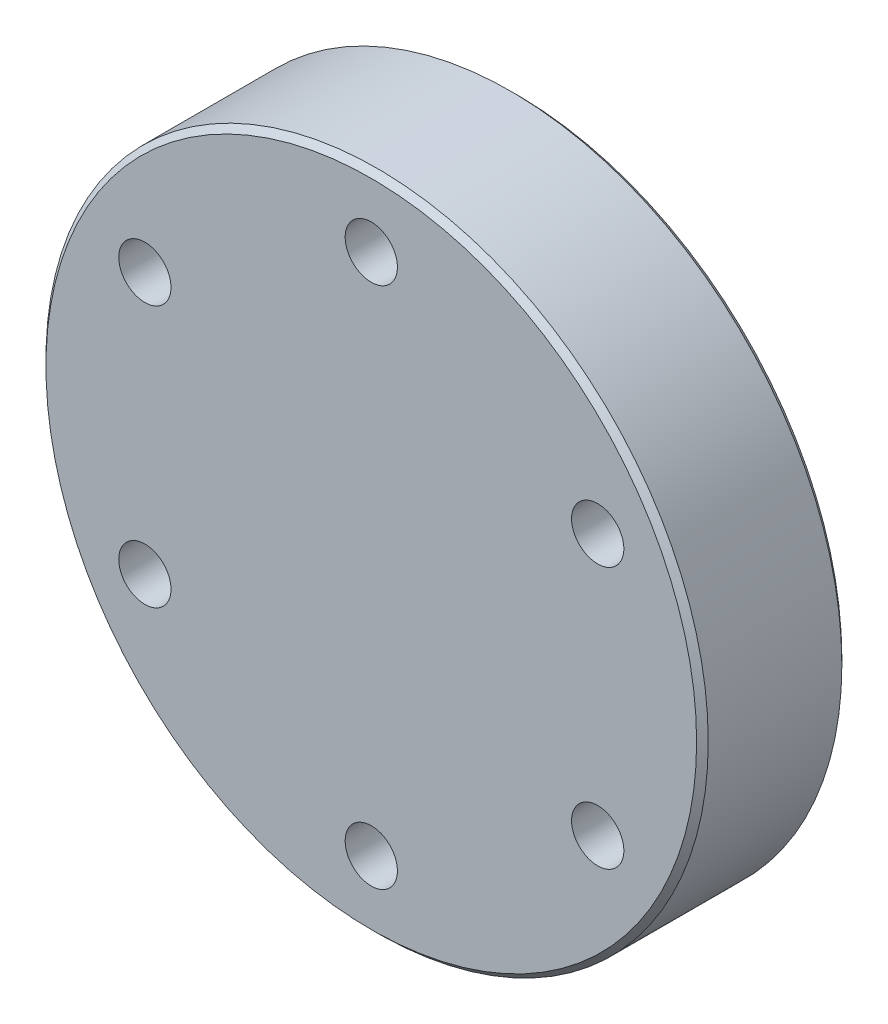
from build123d import *

# Parameters (mm, degrees)
SKETCH1_R                                           = 57
BOSS_EXTRUDE1_DEPTH                                 = 25
CHAMFER3_SIZE                                       = 1
HOLE_SIZE_PER_SOCKET_HEAD_CAP_SCREW_TYP_D           = 9
HOLE_SIZE_PER_SOCKET_HEAD_CAP_SCREW_TYP_CBORE_D     = 15
HOLE_SIZE_PER_SOCKET_HEAD_CAP_SCREW_TYP_CBORE_DEPTH = 12
CIRPATTERN1_COUNT                                   = 6


with BuildPart() as part:
    # Sketch1 → Boss-Extrude1 (new body)
    with BuildSketch(Plane.XY):
        Circle(SKETCH1_R)
    extrude(amount=BOSS_EXTRUDE1_DEPTH)

    # Chamfer3
    chamfer3_edges = [part.edges().sort_by_distance(p)[0] for p in [
        (-57, 0, 0),
        (-57, 0, 25),
    ]]
    chamfer(chamfer3_edges, length=CHAMFER3_SIZE)

    # Hole size (per socket head cap screw type)1 (through all)
    with Locations(Plane(origin=(0, 0, 0), x_dir=(-1, 0, 0), z_dir=(0, 0, -1))):
        with Locations((0, 45)):
            hole_size_per_socket_head_cap_screw_typ = CounterBoreHole(HOLE_SIZE_PER_SOCKET_HEAD_CAP_SCREW_TYP_D / 2, HOLE_SIZE_PER_SOCKET_HEAD_CAP_SCREW_TYP_CBORE_D / 2, HOLE_SIZE_PER_SOCKET_HEAD_CAP_SCREW_TYP_CBORE_DEPTH)

    # CirPattern1: Hole size (per socket head cap screw type)1 ×6 about axis
    cirpattern1_axis = Axis((0, 0, 0), (0, 0, 1))
    for i in range(1, CIRPATTERN1_COUNT):
        add(hole_size_per_socket_head_cap_screw_typ.rotate(cirpattern1_axis, i * 360 / CIRPATTERN1_COUNT), mode=Mode.SUBTRACT)


solid = part.part
